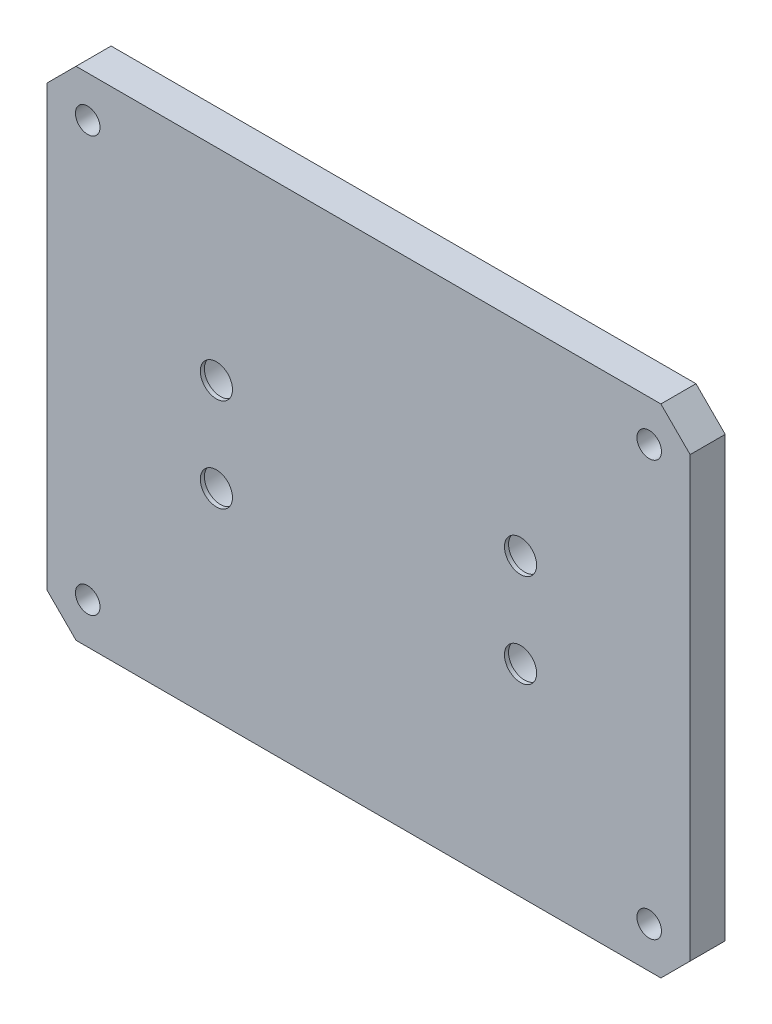
from build123d import *

# Parameters (mm, degrees)
SKETCH_1_W                = 110
SKETCH_1_H                = 85
EXTRUDE_1_DEPTH           = 6
CHAMFER_1_SIZE            = 5
HOLE_WIZARD_1_D           = 5.5
HOLE_WIZARD_1_CBORE_D     = 10
HOLE_WIZARD_1_CBORE_DEPTH = 5.3
HOLE_WIZARD_M5_1_D        = 4.2
HOLE_WIZARD_M5_1_DEPTH    = 12.4
HOLE_WIZARD_M5_1_TIP      = 1.2618073


with BuildPart() as part:
    # 草图1 → 凸台-拉伸1 (new body)
    with BuildSketch(Plane.XY):
        with Locations((-21.033643231, -11.115148183)):
            Rectangle(SKETCH_1_W, SKETCH_1_H)
    extrude(amount=EXTRUDE_1_DEPTH)

    # 倒角1
    chamfer_1_edges = [part.edges().sort_by_distance(p)[0] for p in [
        (-76.033643231, 31.384851817, 3),
        (33.966356769, 31.384851817, 3),
        (33.966356769, -53.615148183, 3),
        (-76.033643231, -53.615148183, 3),
    ]]
    chamfer(chamfer_1_edges, length=CHAMFER_1_SIZE)

    # 打孔尺寸根据内六角圆柱头螺钉的类型1 (through all)
    with Locations(Plane(origin=(0, 0, 0), x_dir=(-1, 0, 0), z_dir=(0, 0, -1))):
        with Locations((47.033643231, -19.115148183), (-4.966356769, -19.115148183), (-4.966356769, -3.115148183), (47.033643231, -3.115148183)):
            CounterBoreHole(HOLE_WIZARD_1_D / 2, HOLE_WIZARD_1_CBORE_D / 2, HOLE_WIZARD_1_CBORE_DEPTH)

    # M5 螺纹孔1
    with Locations(Plane.XY.offset(6)):
        with Locations((-69.033643231, 24.384851817), (26.966356769, 24.384851817), (26.966356769, -46.615148183), (-69.033643231, -46.615148183)):
            Hole(HOLE_WIZARD_M5_1_D / 2, depth=HOLE_WIZARD_M5_1_DEPTH)
            with Locations((0, 0, -(HOLE_WIZARD_M5_1_DEPTH + HOLE_WIZARD_M5_1_TIP / 2))):  # 118° drill point
                Cone(0, HOLE_WIZARD_M5_1_D / 2, HOLE_WIZARD_M5_1_TIP, mode=Mode.SUBTRACT)


solid = part.part
